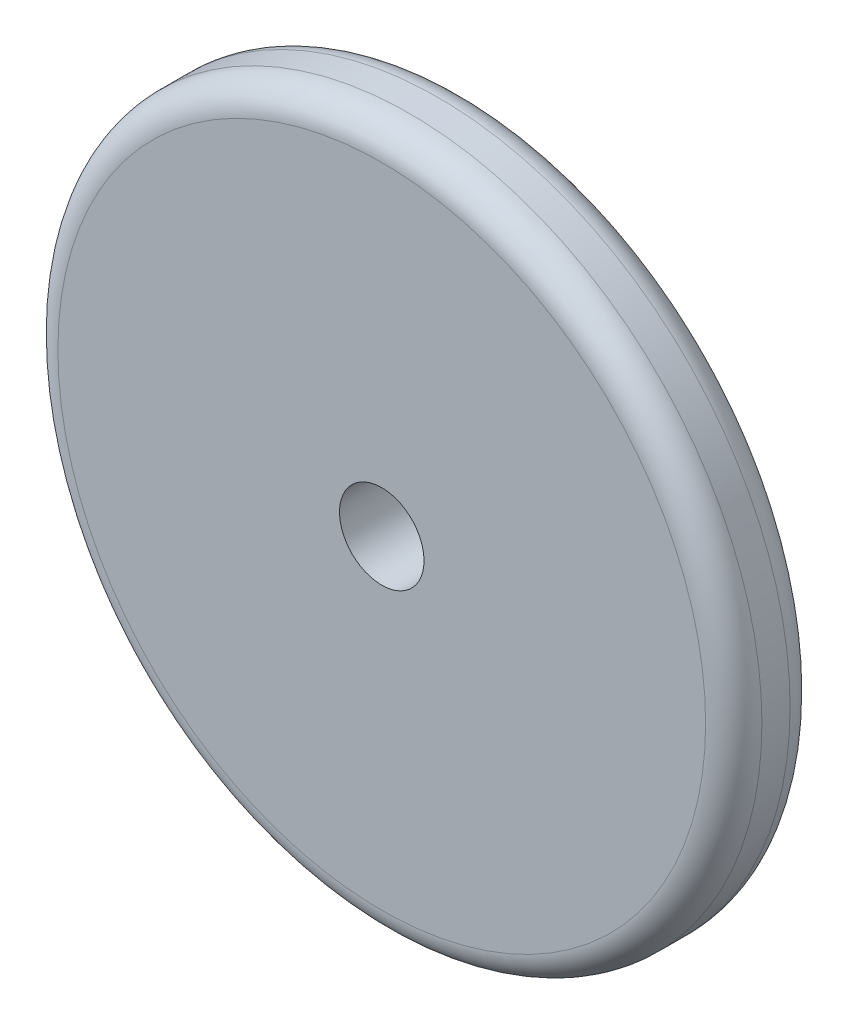
from build123d import *

# Parameters (mm, degrees)
MODEL_R             = 25
MODEL_R_2           = 3
BOSS_EXTRUDE1_DEPTH = 6
FILLET1_R           = 2


with BuildPart() as part:
    # Model → Boss-Extrude1 (new body)
    with BuildSketch(Plane.XY):
        with Locations((-26.872983371, -17.894565392)):
            Circle(MODEL_R)
        with Locations((-26.872983371, -17.894565392)):
            Circle(MODEL_R_2, mode=Mode.SUBTRACT)
    extrude(amount=BOSS_EXTRUDE1_DEPTH)

    # Fillet1
    fillet1_edges = [part.edges().sort_by_distance(p)[0] for p in [
        (-51.872983371, -17.894565392, 0),
        (-51.872983371, -17.894565392, 6),
    ]]
    fillet(fillet1_edges, radius=FILLET1_R)


solid = part.part
